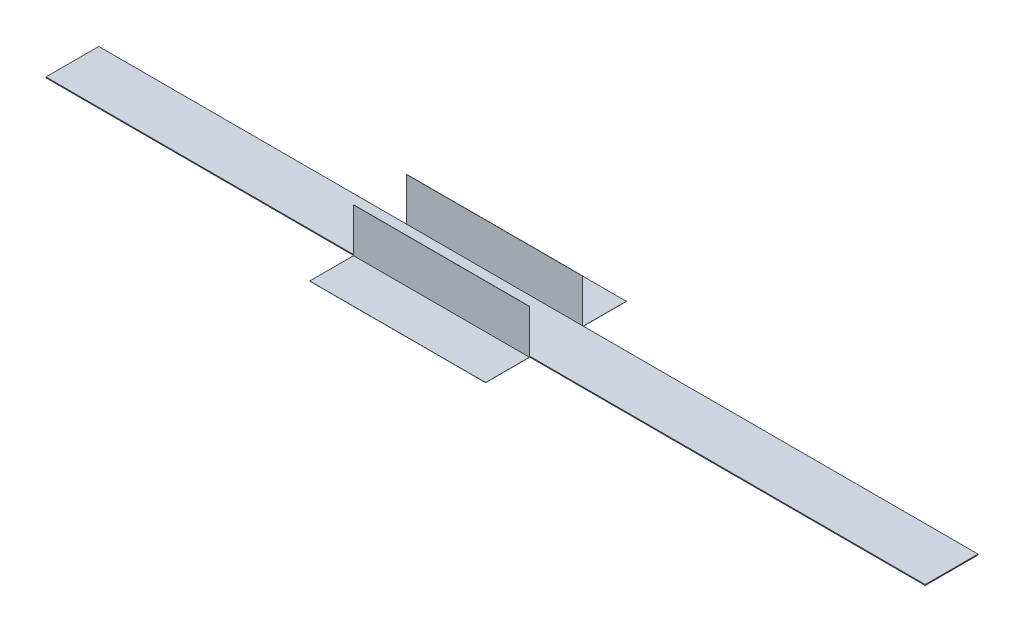
from build123d import *

# Parameters (mm, degrees)
SKETCH1_W           = 100
SKETCH1_H           = 0.1
EXTRUDE_THIN1_DEPTH = 3
SKETCH2_W           = 20
SKETCH2_H           = 16
BOSS_EXTRUDE1_DEPTH = 0.02
SKETCH3_W           = 20
SKETCH3_H           = 0.02
BOSS_EXTRUDE2_DEPTH = 5


with BuildPart() as part:
    # Sketch1 → Extrude-Thin1 (new, symmetric)
    with BuildSketch(Plane.XY):
        with Locations((50, 0)):
            Rectangle(SKETCH1_W, SKETCH1_H)
    extrude(amount=EXTRUDE_THIN1_DEPTH, both=True)

    # Sketch2 → Boss-Extrude1 (add)
    with BuildSketch(Plane.XZ.offset(0.05)):
        with Locations((45, 0)):
            Rectangle(SKETCH2_W, SKETCH2_H)
    extrude(amount=BOSS_EXTRUDE1_DEPTH)

    # Sketch3 → Boss-Extrude2 (add)
    with BuildSketch(Plane(origin=(0, -0.05, 0), x_dir=(1, 0, 0), z_dir=(0, 1, 0))):
        with Locations((45, 3.01)):
            Rectangle(SKETCH3_W, SKETCH3_H)
        with Locations((45, -3.01)):
            Rectangle(SKETCH3_W, SKETCH3_H)
    extrude(amount=BOSS_EXTRUDE2_DEPTH)


solid = part.part
